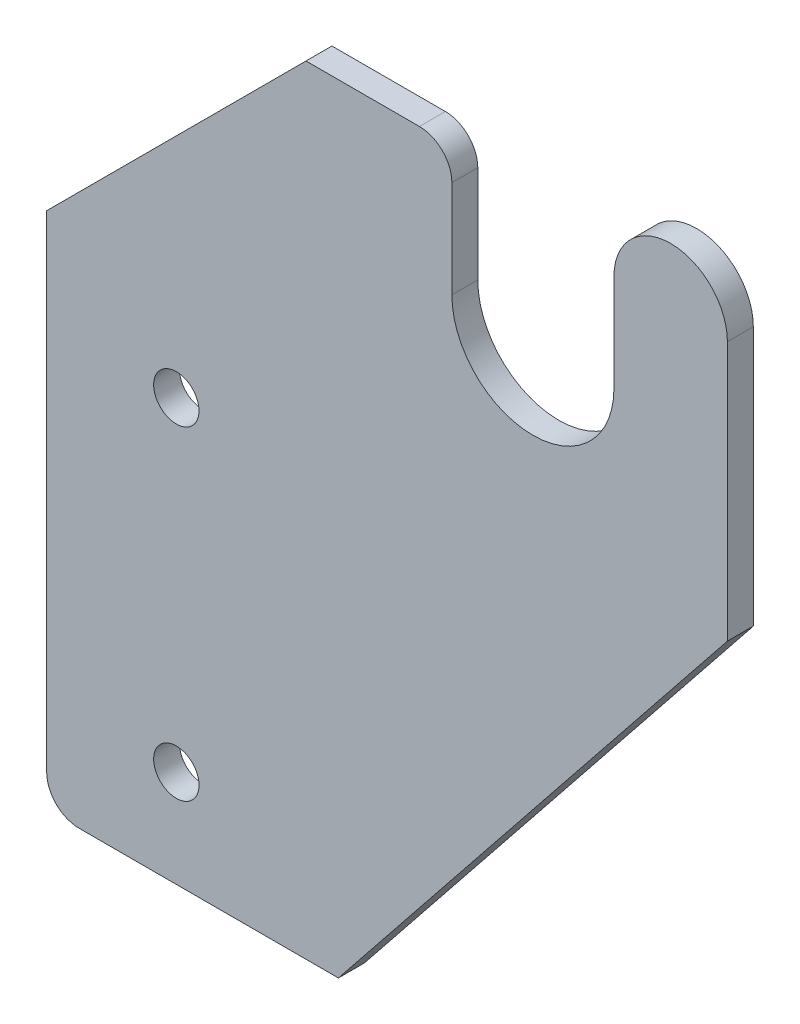
SolidWorks part; units mm, degrees
material "普通碳钢"
ref_plane "Front Plane" through (0, 0, 0) normal (0, 0, 1) x (1, 0, 0)
ref_plane "Top Plane" through (0, 0, 0) normal (0, 1, 0) x (1, 0, 0)
ref_plane "Right Plane" through (0, 0, 0) normal (1, 0, 0) x (0, 0, -1)
sketch "Sketch1" plane through (0, 0, 0) normal (0, 0, 1) x (1, 0, 0)
  line L0 (10, 0) -> (90, 0)
  line L1 (90, 0) -> (210, 150)
  line L2 (210, 150) -> (210, 320) construction
  line L3 (160, 320) -> (210, 320) construction
  line L4 (175, 230) -> (175, 200)
  line L5 (160, 320) -> (160, 240) construction
  line L6 (125, 200) -> (125, 230)
  line L7 (115, 240) -> (80, 240)
  line L8 (80, 240) -> (0, 160)
  line L9 (0, 160) -> (0, 10)
  line L10 (160, 240) -> (165, 240) construction
  line L12 (210, 230) -> (210, 150)
  circle A0 centre (40, 130) radius 7
  circle A1 centre (40, 30) radius 7
  arc A2 (125, 200) -> (175, 200) centre (150, 200) ccw
  arc A3 (10, 0) -> (0, 10) centre (10, 10) cw
  arc A4 (160, 320) -> (160, 240) centre (160, 280) ccw construction
  arc A5 (175, 230) -> (165, 240) centre (165, 230) ccw construction
  arc A6 (125, 230) -> (115, 240) centre (115, 230) ccw
  arc A7 (210, 230) -> (175, 230) centre (192.5, 230) ccw
  point P24 (0, 0)
  point P27 (210, 240)
  dimension "D5" = 14
  dimension "D13" = 10
  dimension "D20" = 5
  dimension "D18" = 10
  dimension "D17" = 50
  dimension "D16" = 10
  dimension "D23" = 35
  dimension "D1" = 50
  dimension "D2" = 90
  dimension "D3" = 40
  dimension "D4" = 30
  dimension "D6" = 240
  dimension "D7" = 160
  dimension "D8" = 150
  dimension "D9" = 150
  dimension "D10" = 210
  dimension "D11" = 80
  dimension "D12" = 200
  dimension "D14" = 100
  dimension "D15" = 170
  dimension "D19" = 35
  dimension "D21" = 80
extrude "Boss-Extrude1" add sketch "Sketch1" along normal blind 8
